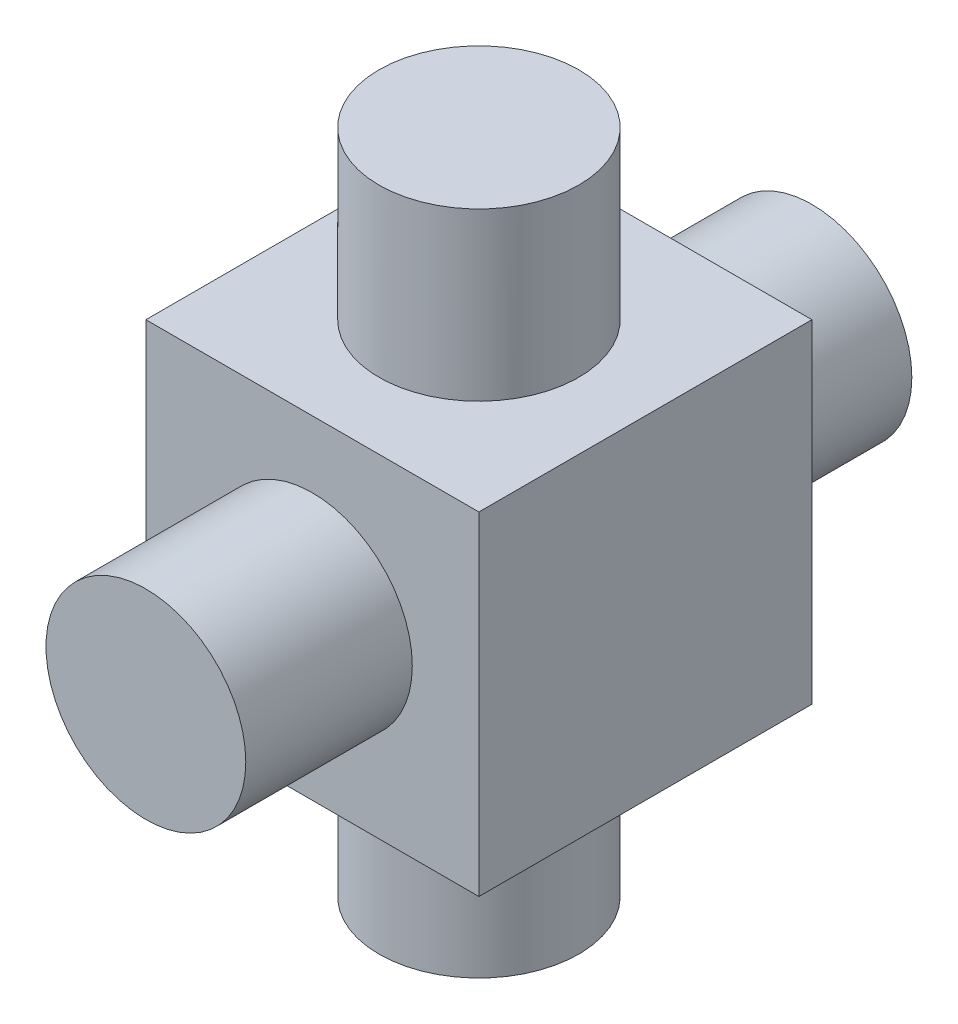
from build123d import *

# Parameters (mm, degrees)
SKETCH_1_W      = 5
SKETCH_1_H      = 5
EXTRUDE_1_DEPTH = 2.5
SKETCH_2_R      = 1.5
EXTRUDE_2_DEPTH = 5
SKETCH_3_R      = 1.5
EXTRUDE_3_DEPTH = 5


with BuildPart() as part:
    # 草图1 → 凸台-拉伸1 (new, symmetric)
    with BuildSketch(Plane.XY):
        Rectangle(SKETCH_1_W, SKETCH_1_H)
    extrude(amount=EXTRUDE_1_DEPTH, both=True)

    # 草图2 → 凸台-拉伸2 (add, symmetric)
    with BuildSketch(Plane(origin=(0, 0, 0), x_dir=(1, 0, 0), z_dir=(0, 1, 0))):
        with Locations(Location((0, 0, 0), (0, 0, 90))):
            Circle(SKETCH_2_R)
    extrude(amount=EXTRUDE_2_DEPTH, both=True)

    # 草图3 → 凸台-拉伸3 (add, symmetric)
    with BuildSketch(Plane.XY):
        Circle(SKETCH_3_R)
    extrude(amount=EXTRUDE_3_DEPTH, both=True)


solid = part.part
